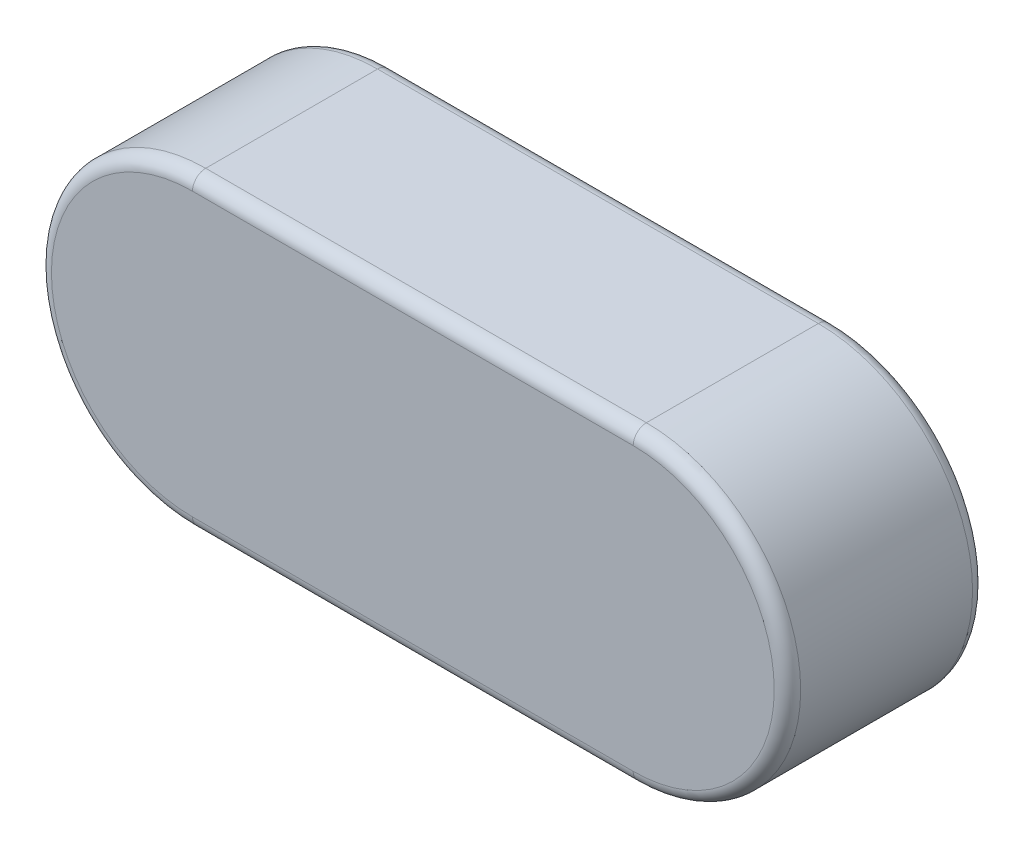
SolidWorks part; units mm, degrees
ref_plane "基准面1" through (0, 0, 0) normal (0, 0, 1) x (1, 0, 0)
ref_plane "基准面2" through (0, 0, 0) normal (0, 1, 0) x (1, 0, 0)
ref_plane "基准面3" through (0, 0, 0) normal (1, 0, 0) x (0, 0, -1)
sketch "尺寸草图" plane through (0, 0, 0) normal (0, 0, 1) x (1, 0, 0)
  line L0 (-17, 0) -> (17, 0) construction
  point P3 (-9, 0)
  point P4 (-0.6, 0)
  point P5 (0, 0)
  point P8 (-14, 0)
  point P11 (0, 0)
sketch "草图1" plane through (0, 0, 0) normal (0, 0, 1) x (1, 0, 0)
  line L0 (-28.0599, 0) -> (30.562, 0) construction
  line L1 (-10, 7) -> (10, 7)
  line L2 (-10, -7) -> (10, -7)
  line L3 (0, 2.9108) -> (0, -2.1805) construction
  arc A0 (-10, 7) -> (-10, -7) centre (-10, 0) ccw
  arc A1 (10, 7) -> (10, -7) centre (10, 0) cw
extrude "基体-拉伸" add sketch "草图1" along normal blind 9
fillet "圆角1" radius 0.6 8 edges at (17, 0, 9) (0, 7, 9) (-17, 0, 9) (0, 7, 0) (17, 0, 0) (0, -7, 0) (-17, 0, 0) (0, -7, 9)
equation "\"D3@草图1\" = \"L@尺寸草图\""
equation "\"D1@草图1\" = \"b@尺寸草图\" / 2"
equation "\"D1@圆角1\" = \"r@尺寸草图\""
equation "\"D1@基体-拉伸\" = \"h@尺寸草图\""
